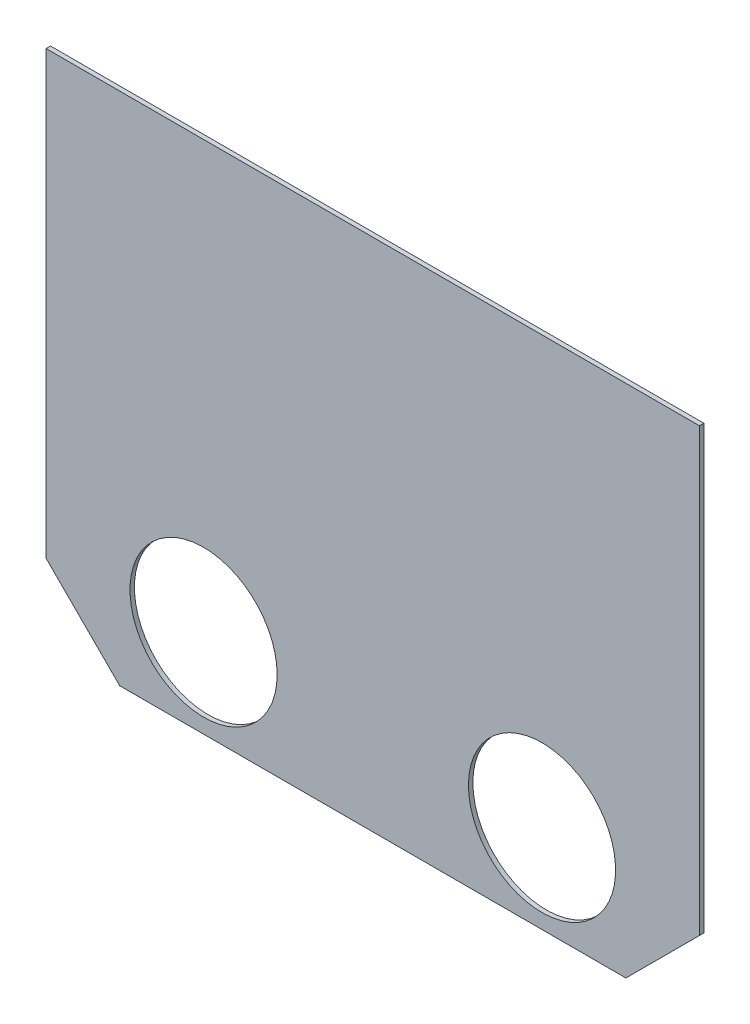
SolidWorks part; units mm, degrees
material "Q235A"
ref_plane "Front Plane" through (0, 0, 0) normal (0, 0, 1) x (1, 0, 0)
ref_plane "Top Plane" through (0, 0, 0) normal (0, 1, 0) x (1, 0, 0)
ref_plane "Right Plane" through (0, 0, 0) normal (1, 0, 0) x (0, 0, -1)
sketch "Sketch1" plane through (0, 0, 0) normal (0, 0, 1) x (1, 0, 0)
  line L0 (222, 0) -> (222, 350) construction
  line L1 (50, 0) -> (394, 0)
  line L2 (0, 50) -> (0, 350)
  line L3 (0, 350) -> (444, 350)
  line L4 (444, 50) -> (394, 0)
  line L5 (0, 50) -> (50, 0)
  line L6 (444, 50) -> (444, 350)
  circle A0 centre (107, 60) radius 50
  circle A1 centre (337, 60) radius 50
  point P0 (0, 0)
  point P7 (444, 0)
  dimension "D3" = 100
  dimension "D4" = 222
  dimension "D7" = 60
  dimension "D8" = 115
  dimension "D2" = 350
extrude "Boss-Extrude1" add sketch "Sketch1" along normal mid plane 3
